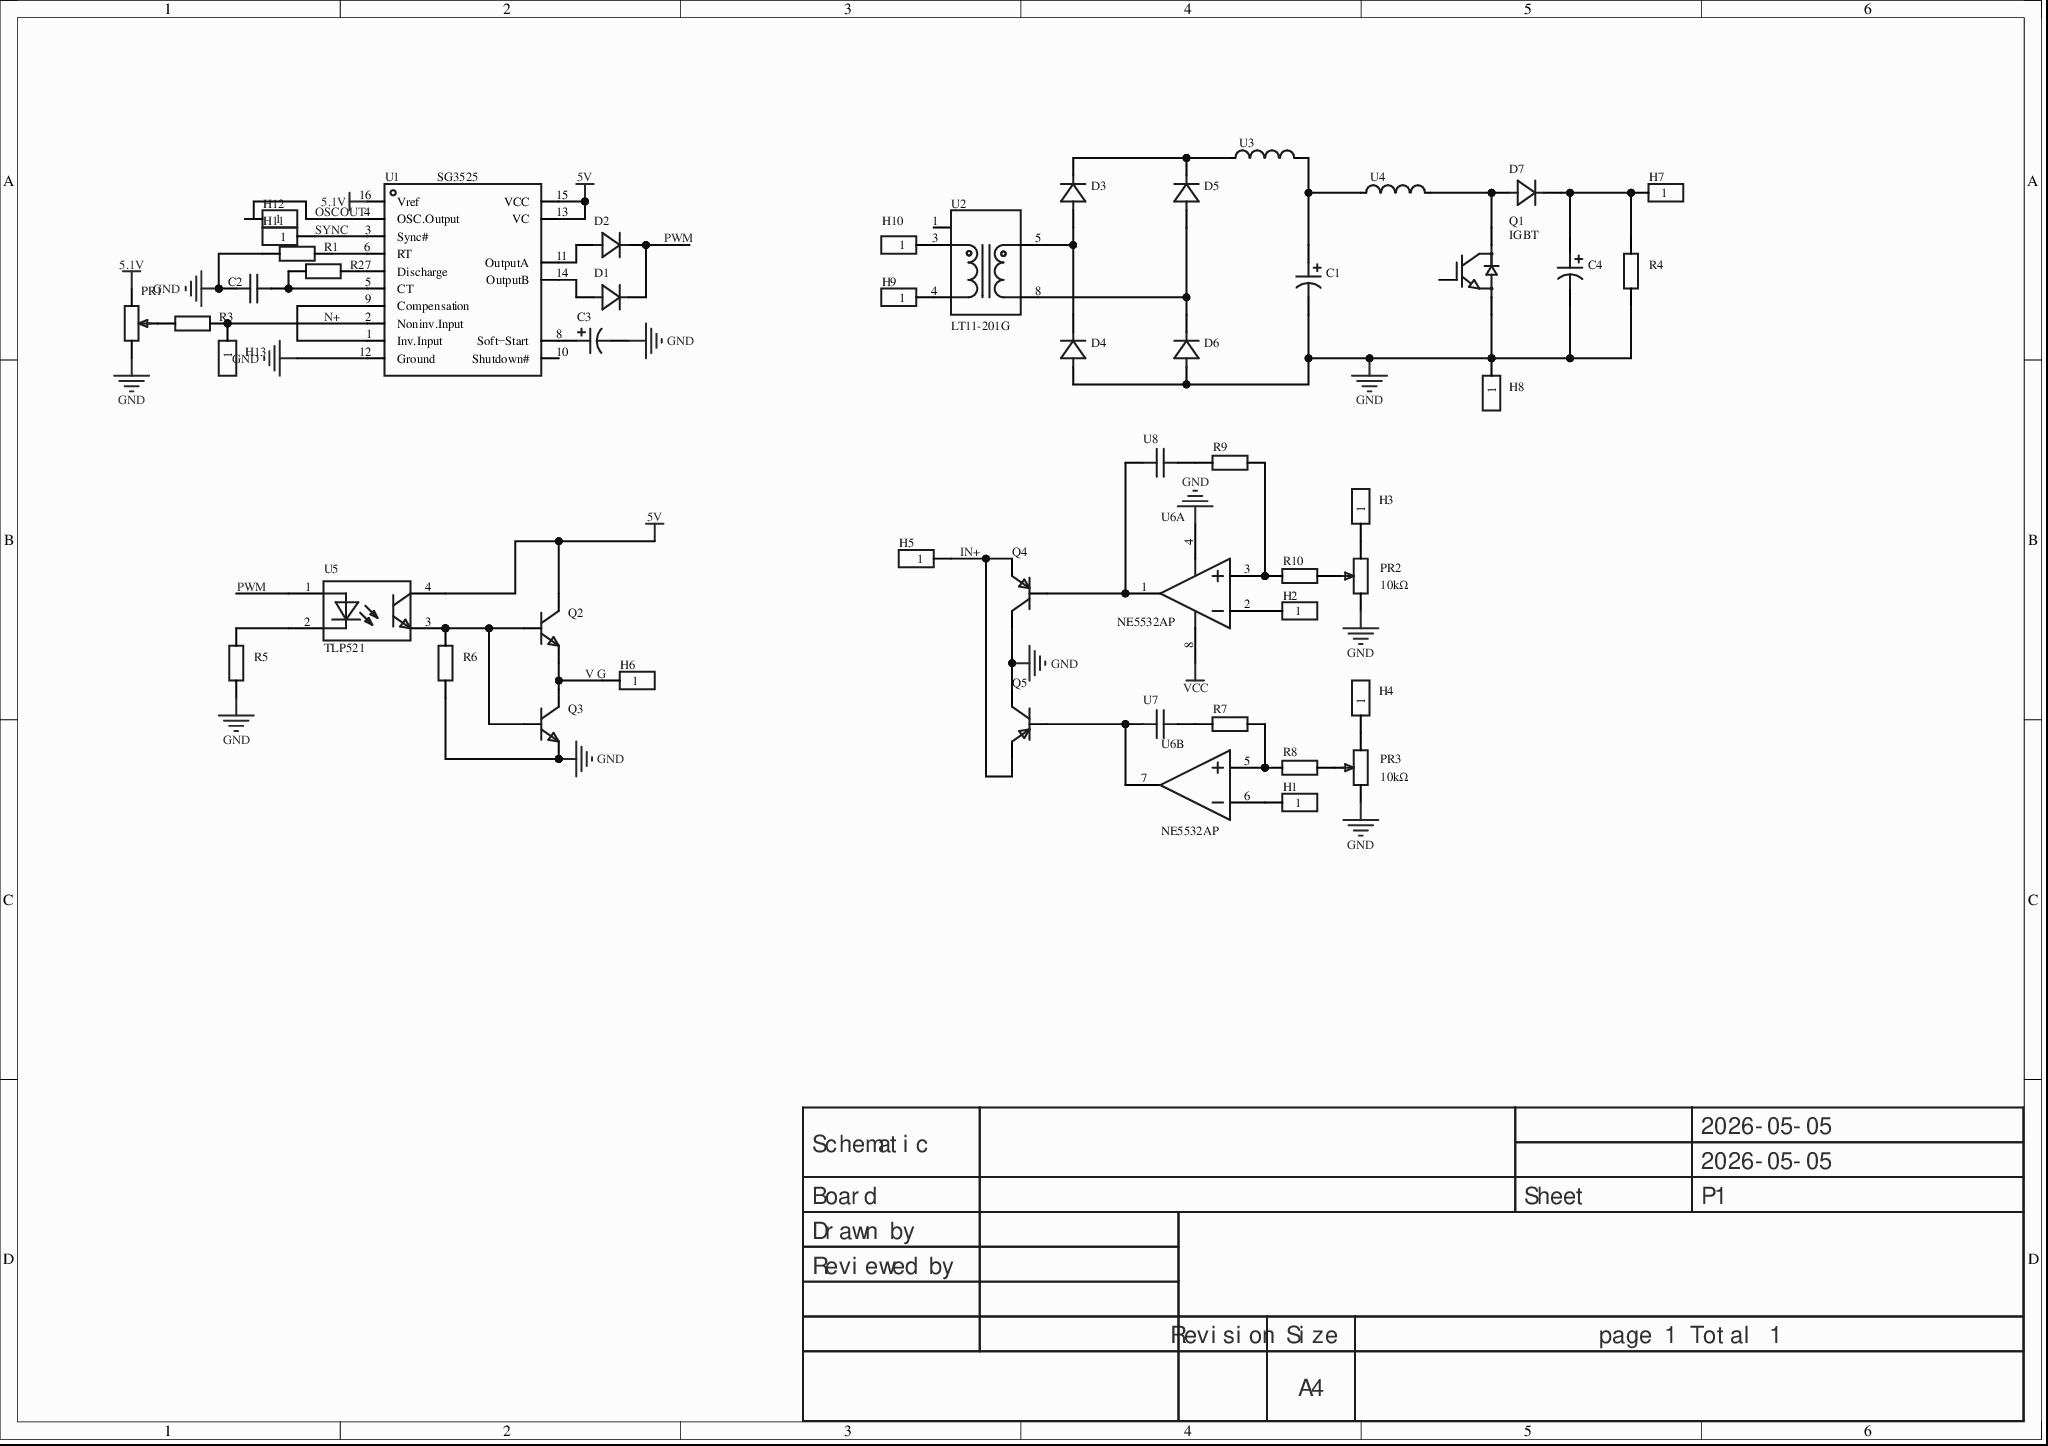
[diagram p0: MISC51628-3.schdoc]
# Altium project MISC51628-2.PrjPcb
1 sheet, 50 parts. Net scope: global (net labels, ports and power ports of the same name join across sheets).
Board file: MISC51628.pcbdoc

## Sheet MISC51628-3.schdoc
size 297 x 209 mm; Version: V1.0; @Project Name: MISC51628; @Update Date: 2026-05-05; @Create Date: 2026-05-05; @Board Name: MISC51628; @Create Time: 00:14:23; @Page Count: 1; @Page No: 1; @Schematic Name: MISC51628; @Update Time: 00:14:23; Size: A4

### Parts
C1  10uF  [CAP-TH_BD5.0-P2.00-D0.8-FD-10UF50VC110GL]  (value not drawn)
C2  100nF  [CAP-TH_L5.0-W2.5-P5.00-D1.0]  (value not drawn)
C3  10uF  [CAP-TH_BD5.0-P2.00-D0.8-FD-10UF50VC110GL]  (value not drawn)
C4  10uF  [CAP-TH_BD5.0-P2.00-D0.8-FD-10UF50VC110GL]  (value not drawn)
D1  (no value)  [DO_1N4007]
D2  (no value)  [DO_1N4007]
D3  (no value)  [DO_1N4007]
D4  (no value)  [DO_1N4007]
D5  (no value)  [DO_1N4007]
D6  (no value)  [DO_1N4007]
D7  (no value)  [DO_1N4007]
H1  (no value)  [HDR-TH_1P-V-M_XKB_X4611WV-01I-C28D40]
H2  (no value)  [HDR-TH_1P-V-M_XKB_X4611WV-01I-C28D40]
H3  (no value)  [HDR-TH_1P-V-M_XKB_X4611WV-01I-C28D40]
H4  (no value)  [HDR-TH_1P-V-M_XKB_X4611WV-01I-C28D40]
H5  (no value)  [HDR-TH_1P-V-M_XKB_X4611WV-01I-C28D40]
H6  (no value)  [HDR-TH_1P-V-M_XKB_X4611WV-01I-C28D40]
H7  (no value)  [HDR-TH_1P-V-M_XKB_X4611WV-01I-C28D40]
H8  (no value)  [HDR-TH_1P-V-M_XKB_X4611WV-01I-C28D40]
H9  (no value)  [HDR-TH_1P-V-M_XKB_X4611WV-01I-C28D40]
H10  (no value)  [HDR-TH_1P-V-M_XKB_X4611WV-01I-C28D40]
H11  (no value)  [HDR-TH_1P-V-M_XKB_X4611WV-01I-C28D40]
H12  (no value)  [HDR-TH_1P-V-M_XKB_X4611WV-01I-C28D40]
H13  (no value)  [HDR-TH_1P-V-M_XKB_X4611WV-01I-C28D40]
PR1  10kΩ  [R_3296]  (value not drawn)
PR2  10kΩ  [R_3296]
PR3  10kΩ  [R_3296]
Q1  IGBT  [TO-247-3_L15.9-W5.0-P5.44-L]
Q2  (no value)  [S8050_TO_92]
Q3  (no value)  [S8050_TO_92]
Q4  (no value)  [S8550P_SOT]
Q5  (no value)  [S8550P_SOT]
R1  10kΩ  [Res_1/8W]  (value not drawn)
R2  10kΩ  [Res_1/8W]  (value not drawn)
R3  10kΩ  [Res_1/8W]  (value not drawn)
R4  10kΩ  [Res_1/8W]  (value not drawn)
R5  10kΩ  [Res_1/8W]  (value not drawn)
R6  10kΩ  [Res_1/8W]  (value not drawn)
R7  10kΩ  [Res_1/8W]  (value not drawn)
R8  10kΩ  [Res_1/8W]  (value not drawn)
R9  10kΩ  [Res_1/8W]  (value not drawn)
R10  10kΩ  [Res_1/8W]  (value not drawn)
U1  SG3525  [DIP-16_L19.2-W6.6-P2.54-LS7.6-BL]
U2  LT11-201G  [XFMR-TH_LT13-201]
U3  Power inductor (SMD), CKST0502-10uH/M, 10uH, ±20%, 3A, package 5.7mm*5.1mm*2.0mm, Cenke, RoHS  [IND-SMD_L5.7-W5.1]  (value not drawn)
U4  Power inductor (SMD), CKST0502-10uH/M, 10uH, ±20%, 3A, package 5.7mm*5.1mm*2.0mm, Cenke, RoHS  [IND-SMD_L5.7-W5.1]  (value not drawn)
U5  TLP521  [SOP-4_L6.4-W4.6-P2.54-LS10.2-TL]
U6  NE5532AP  [PDIP-8_L9.6-W6.4-P2.54-LS7.6-BL]  (parts A,B of 2)
U7  100nF  [CAP-TH_L5.0-W2.5-P5.00-D1.0]  (value not drawn)
U8  100nF  [CAP-TH_L5.0-W2.5-P5.00-D1.0]  (value not drawn)

### Nets
5.1V: PR1.3 U1.16(Vref)
5V: Q2.3(C) U1.13(VC) U1.15(VCC) U5.4
GND: C1.2 C2.2 C3.2 C4.2 D4.2(A) D6.2(A) H8.1 PR1.1 PR2.3 PR3.3 Q1.3(E) Q3.1(E) Q4.3(C) Q5.3(C) R1.1 R4.1 R5.1 R6.1 U1.12(Ground) U6.4(V-)
VCC: U6.8(V+)
IN+: H5.1 Q4.2(E) Q5.2(E)
N+: H13.1 R3.2 U1.2(Noninv.Input)
OSCOUT: H12.1 U1.4(OSC.Output)
PWM: D1.1(K) D2.1(K) U5.1
SYNC: H11.1 U1.3(Sync#)
V G: H6.1 Q2.1(E) Q3.3(C)
NetC1_1: C1.1 U3.2 U4.1
NetC2_1: C2.1 R2.1 U1.5(CT)
NetC3_1: C3.1 U1.8(Soft−Start)
NetC4_1: C4.1 D7.1(K) H7.1 R4.2
NetD1_2: D1.2(A) U1.14(OutputB)
NetD2_2: D2.2(A) U1.11(OutputA)
NetD3_1: D3.1(K) D5.1(K) U3.1
NetD3_2: D3.2(A) D4.1(K) U2.5
NetD5_2: D5.2(A) D6.1(K) U2.8
NetD7_2: D7.2(A) Q1.2(C) U4.2
NetH1_1: H1.1 U6.6(IN_B-)
NetH2_1: H2.1 U6.2(IN_A-)
NetH3_1: H3.1 PR2.1
NetH4_1: H4.1 PR3.1
NetH9_1: H9.1 U2.4
NetH10_1: H10.1 U2.3
NetPR1_2: PR1.2 R3.1
NetPR2_2: PR2.2 R10.1
NetPR3_2: PR3.2 R8.1
NetQ2_2: Q2.2(B) Q3.2(B) R6.2 U5.3
NetQ4_1: Q4.1(B) U6.1(OUT_A) U8.2
NetQ5_1: Q5.1(B) U6.7(OUT_B) U7.2
NetR1_2: R1.2 U1.6(RT)
NetR2_2: R2.2 U1.7(Discharge)
NetR5_2: R5.2 U5.2
NetR7_1: R7.1 R8.2 U6.5(IN_B+)
NetR7_2: R7.2 U7.1
NetR9_1: R9.1 R10.2 U6.3(IN_A+)
NetR9_2: R9.2 U8.1
NetU1_1: U1.1(Inv.Input) U1.9(Compensation)

Not connected (* = marked no-connect by the designer): Q1 1(G); U1 10(Shutdown#); U2 1

### Notes on the sheet
- 2026-05-05
- Schematic
- Board
- Sheet
- P1
- Drawn by
- Reviewed by
- Revision
- Size
- A4
- page 1 Total 1

### Library data of the parts
C1 C4 = 10UF50VC110GL: Capacitance:10uF;Tolerance:±20%;Rated voltage:50V;Ripple current:120mA@100KHz;Equivalent series resistance(ESR):1.6Ω;; Manufacturer: Econd(米朗电子); Tolerance: ±20%; Voltage Rating: 50V; Equivalent Series Resistance(ESR): 1.6Ω; Pin Spacing: 2mm; Lifetime: 5000hrs@105℃; AddInBom: yes; Symbol: 10UF50VC110GL; Device: 10UF50VC110GL; LCSC Part Name: 10uF ±20% 50V; Supplier Part: C46867109; Manufacturer Part: 10UF50VC110GL; Supplier Footprint: 插件,D5xL11mm; JLCPCB Part Class: Extended Part; Datasheet: https://example.com/datasheet/10UF50VC110GL/49031974.html; Supplier: LCSC; Value: 10uF; Ripple Current: 120mA@100KHz; Diameter: 5mm; Height - Seated (Max): 11mm; Operating Temperature: -40℃~+105℃; ConvertToPcb: yes; FootprintName: CAP-TH_BD5.0-P2.00-D0.8-FD-10UF50VC110GL
C2 = 100nF: Symbol: 100NF_C9900015256; AddInBom: yes; ModelId: 08e3d7481fc7486bb1b263873f51e1e10819f05c4eef4c71ace90d822a990e87; ModelName: CAP-TH_BD5.0-W2.5-P5.08; ModelTransform: 224.652,98.425,0,0,0,0,-0.005,0,-137.795; Device: 100nF; LCSC Part Name: 100nF; SupplierPart: C9900015256; ManufacturerPart: 100nF; Supplier Footprint: CAP-TH_L5.0-W2.5-P5.00-D1.0; JLCPCB Part Class: Extended Part; Supplier: LCSC; ConvertToPcb: yes; FootprintName: CAP-TH_L5.0-W2.5-P5.00-D1.0
C3 = 10UF50VC110GL: Capacitance:10uF;Tolerance:±20%;Rated voltage:50V;Ripple current:120mA@100KHz;Equivalent series resistance(ESR):1.6Ω;; Manufacturer: Econd(米朗电子); AddInBom: yes; Tolerance: ±20%; Voltage Rating: 50V; Equivalent Series Resistance(ESR): 1.6Ω; Pin Spacing: 2mm; Lifetime: 5000hrs@105℃; Symbol: 10UF50VC110GL; Device: 10UF50VC110GL; LCSC Part Name: 10uF ±20% 50V; SupplierPart: C46867109; ManufacturerPart: 10UF50VC110GL; Supplier Footprint: 插件,D5xL11mm; JLCPCB Part Class: Extended Part; Datasheet: https://example.com/datasheet/10UF50VC110GL/49031974.html; Supplier: LCSC; ConvertToPcb: yes; FootprintName: CAP-TH_BD5.0-P2.00-D0.8-FD-10UF50VC110GL; Value: 10uF; Ripple Current: 120mA@100KHz; Diameter: 5mm; Height - Seated (Max): 11mm; Operating Temperature: -40℃~+105℃
D1-D3 = D_1N4007A: AddInBom: yes; ModelId: 6de1e9b71a0d4751b4e9df530304c1a30819f05c4eef4c71ace90d822a990e87; ModelName: DO-41_D2.4-L4.7-P8.70; ModelTransform: 373.9,94.4,232.29,0,0,0,0,0,-140; Symbol: D_1N4007; Device: D_1N4007A; Supplier Footprint: DO-41; ConvertToPcb: yes; FootprintName: DO_1N4007
D4-D7 = D_1N4007A: 3D Model: 6de1e9b71a0d4751b4e9df530304c1a30819f05c4eef4c71ace90d822a990e87; 3D Model Transform: 373.9,94.4,232.29,0,0,0,0,0,-140; AddInBom: yes; ModelName: DO-41_D2.4-L4.7-P8.70; Symbol: D_1N4007; Device: D_1N4007A; Supplier Footprint: DO-41; ConvertToPcb: yes; FootprintName: DO_1N4007
H1-H13 = HDR-M_2.54_1x1P: Symbol: HDR_1x1; ConvertToPcb: yes; ModelId: 95857080d3cc4057a19a22ccce05e1710819f05c4eef4c71ace90d822a990e87; ModelTransform: 78.74,79.1337,0,0,0,0,0,0,-110.236; Device: HDR-M_2.54_1x1P; AddInBom: yes; SupplierPart: C81276; Supplier Footprint: 插件; FootprintName: HDR-TH_1P-V-M_XKB_X4611WV-01I-C28D40; JLCPCB Part Class: Extended Part; ModelName: HDR-TH_1P-V-M_XKB_X4611WV-01I-C28D40
PR1 = R_3296: ConvertToPcb: yes; ModelId: b182808559bb43bda9e7de64b64134cb0819f05c4eef4c71ace90d822a990e87; ModelName: 3296W; ModelTransform: 373.98,188.96,590.49,180,0,0,0,0,-140; Symbol: R_3296; Device: R_3296; AddInBom: yes; Supplier Footprint: 直插; FootprintName: R_3296; Value: 10kΩ
PR2 PR3 = R_3296: 3D Model: b182808559bb43bda9e7de64b64134cb0819f05c4eef4c71ace90d822a990e87; 3D Model Transform: 373.98,188.96,590.49,180,0,0,0,0,-140; ConvertToPcb: yes; ModelName: 3296W; Symbol: R_3296; Device: R_3296; Supplier Footprint: 直插; Value: 10kΩ; AddInBom: yes; FootprintName: R_3296
Q1 = MLG40T65FDL-W: Uses advanced trench gate field-stop technology (Trench FS), collector-emitter breakdown voltage Vces=650V, collector current Ic=40A, with low conduction voltage drop and low turn-off loss, etc…; Manufacturer: minos(迈诺斯); AddInBom: yes; ModelId: 06d11a66e67643458860efec572770e60819f05c4eef4c71ace90d822a990e87; ModelTransform: 625.983,196.85,0,0,0,0,0,5.906,-196.85; Symbol: MLG40T65FDL-W; Device: MLG40T65FDL-W; Manufacturer Part: IGBT; LCSC Part Name: IGBT 650V 40A; SupplierPart: C54770473; Supplier Footprint: TO-3P; JLCPCB Part Class: Extended Part; Datasheet: https://example.com/datasheet/MLG40T65FDL-W/58189658.html; Supplier: LCSC; ConvertToPcb: yes; FootprintName: TO-247-3_L15.9-W5.0-P5.44-L; ModelName: TO-247-3_L15.9-W5.0-P5.44-L
Q2 Q3 = S8050_TO_NPN: ConvertToPcb: yes; ModelId: aafe8e06f2154e7c93506efd0d6632dd0819f05c4eef4c71ace90d822a990e87; ModelName: TO-92-3_L4.9-W3.7-P1.27-L; ModelTransform: 180.78,141.44,417.3,0,0,0,0,0,-200; Symbol: S8050_TO_NPN; Device: S8050_TO_NPN; AddInBom: yes; Supplier Footprint: TO-92; FootprintName: S8050_TO_92
Q4 Q5 = S8550_SOT_PNP: Symbol: PNP; ConvertToPcb: yes; ModelId: 9c0df02d6f3e44e889da37f3e5bf54960819f05c4eef4c71ace90d822a990e87; ModelName: SOT-23-3_L2.9-W1.4-P1.90-LS2.5-BR; ModelTransform: 98.43,114.17,37.91,0,0,0,0,0,0; Device: S8550_SOT_PNP; AddInBom: yes; Supplier Footprint: SOT-23; FootprintName: S8550P_SOT
R1-R3 = Res_AXIAL-1/8W: Symbol: Resistor; ConvertToPcb: yes; ModelId: b2b5ae7ae4c642178fe0039925c86a3f0819f05c4eef4c71ace90d822a990e87; ModelName: RES-TH_BD1.8-L3.2-P7.20-D0.4; ModelTransform: 282.86,66.88,253.09,0,0,0,0,0,-191; Device: Res_AXIAL-1/8W; AddInBom: yes; Supplier Footprint: 轴向引线; Value: 10kΩ; FootprintName: Res_1/8W
R4-R10 = Res_AXIAL-1/8W: Symbol: Resistor; 3D Model: b2b5ae7ae4c642178fe0039925c86a3f0819f05c4eef4c71ace90d822a990e87; 3D Model Transform: 282.86,66.88,253.09,0,0,0,0,0,-191; ConvertToPcb: yes; ModelName: RES-TH_BD1.8-L3.2-P7.20-D0.4; Device: Res_AXIAL-1/8W; Supplier Footprint: 轴向引线; Value: 10kΩ; AddInBom: yes; FootprintName: Res_1/8W
U1 = SG3525: Operating voltage: 8V~35V; switching frequency: 100Hz~500kHz; output current: 400mA; transistor withstand voltage: -;; Manufacturer: Gcore(扬州国芯); Symbol: SG3525_1; AddInBom: yes; ModelId: 36ad9a7692634580875d8a15b0e444ee0819f05c4eef4c71ace90d822a990e87; ModelName: DIP-16_L19.2-W6.6-H3.3-LS7.62-P2.54; ModelTransform: 755.904,311.8104,0,0,0,0,0,0,-118.11; Pd - Power Dissipation: 1000mW; Duty Cycle(Max): 49%; Topology: Totem pole; Device: SG3525; LCSC Part Name: PWM控制器; SupplierPart: C5157689; ManufacturerPart: SG3525; Supplier Footprint: DIP-16; JLCPCB Part Class: Extended Part; Datasheet: https://example.com/datasheet/SG3525/5796617.html; Supplier: LCSC; ConvertToPcb: yes; FootprintName: DIP-16_L19.2-W6.6-P2.54-LS7.6-BL; Isolation: -; Voltage - Supply: 8V~35V; Frequency - Switching: 100Hz~500kHz; Output Current: 400mA; Voltage - Breakdown: -; Features: Undervoltage protection (UVP); soft start; Operating Temperature: 0℃~+70℃; Working Mode: -; Output Voltage: -; Feedback System: -
U2 = LT11-201G: Transformer  Through-hole broadband carrier coupling transformer, high withstand voltage; Manufacturer: Linekey(立凯电控); AddInBom: yes; ModelId: 978c4cfc96044b13b294b69b1fbf46df0819f05c4eef4c71ace90d822a990e87; ModelTransform: 399.6055,451.1802,0,0,0,0,-0.002,0,-137.795; Symbol: LT11-201G; Device: LT11-201G; LCSC Part Name: 变压器; SupplierPart: C19274033; ManufacturerPart: LT11-201G; Supplier Footprint: 插件,11.4x10.1mm; JLCPCB Part Class: Extended Part; Datasheet: https://example.com/upload/public/pdf/source/20231201/8CB723A30866AEEAB4FA21B3FDB2AC71.pdf; Supplier: LCSC; ConvertToPcb: yes; FootprintName: XFMR-TH_LT13-201; ModelName: XFMR-TH_LT13-201
U3 U4 = 功率电感(贴片),CKST0502-10uH/M,10uH,±20%,3A,封装5.7mm*5.1mm*2.0mm,岑科,RoHS: AddInBom: yes; ModelId: ffd856615f974dd9b1ff3f65e3b3100d0819f05c4eef4c71ace90d822a990e87; ModelTransform: 224.409,200.787,0,0,0,0,0,-0.591,0; Symbol: Power inductor (SMD), CKST0502-10UH/M, 10UH, ±20%, 3A, package 5.7MM*5.1MM*2.0MM, Cenke, ROHS; Device: Power inductor (SMD), CKST0502-10uH/M, 10uH, ±20%, 3A, package 5.7mm*5.1mm*2.0mm, Cenke, RoHS; LCSC Part Name: 功率电感(贴片),CKST0502-10uH/M,10uH,±20%,3A,封装5.7mm*5.1mm*2.0mm,岑科,RoHS; SupplierPart: C9900015114; ManufacturerPart: 功率电感(贴片),CKST0502-10uH/M,10uH,±20%,3A,封装5.7mm*5.1mm*2.0mm,岑科,RoHS; Supplier Footprint: 功率电感(贴片),CKST0502-10uH/M,10uH,±20%,3A,封装5.7mm*5.1mm*2.0mm,岑科,RoHS; JLCPCB Part Class: Extended Part; Supplier: LCSC; ConvertToPcb: yes; FootprintName: IND-SMD_L5.7-W5.1; ModelName: IND-SMD_L5.7-W5.1
U5 = TLP521: AddInBom: yes; ModelId: 96de0c972fa141a0bf05d1bdcf0ddf4e0819f05c4eef4c71ace90d822a990e87; ModelName: SOP-4_L4.6-W6.5-H3.5-LS10.2_P2.54; ModelTransform: 181.102,401.574,0,270,0,0,0,0,0; Symbol: TLP521; Device: TLP521; LCSC Part Name: TLP521; SupplierPart: C9900005355; ManufacturerPart: TLP521; Supplier Footprint: SOP-4-2.54mm; JLCPCB Part Class: Extended Part; Supplier: LCSC; ConvertToPcb: yes; FootprintName: SOP-4_L6.4-W4.6-P2.54-LS10.2-TL
U6 = NE5532AP: Dual-channel, 30V, 10MHz, low-noise (6nV/√Hz) operational amplifier for audio applications; Manufacturer: TI(德州仪器); Relevance: []; AddInBom: yes; ModelId: 5dc2af053da0476fab11ee64b9a10a940819f05c4eef4c71ace90d822a990e87; ModelName: PDIP-8_L9.6-W6.4-P2.54-LS7.62-BL; ModelTransform: 377.952,309.842,0,0,0,0,0,0,-137.795; Symbol: NE5532AP; Device: NE5532AP; LCSC Part Name: NE5532AP; SupplierPart: C353150; ManufacturerPart: NE5532AP; Supplier Footprint: PDIP-8; JLCPCB Part Class: Extended Part; Supplier: LCSC; ConvertToPcb: yes; FootprintName: PDIP-8_L9.6-W6.4-P2.54-LS7.6-BL
U7 U8 = 100nF: Symbol: 100NF_C9900015256; 3D Model: 08e3d7481fc7486bb1b263873f51e1e10819f05c4eef4c71ace90d822a990e87; 3D Model Transform: 224.652,98.425,0,0,0,0,-0.005,0,-137.795; AddInBom: yes; ModelName: CAP-TH_BD5.0-W2.5-P5.08; Device: 100nF; LCSC Part Name: 100nF; Supplier Part: C9900015256; Manufacturer Part: 100nF; Supplier Footprint: CAP-TH_L5.0-W2.5-P5.00-D1.0; JLCPCB Part Class: Extended Part; Supplier: LCSC; ConvertToPcb: yes; FootprintName: CAP-TH_L5.0-W2.5-P5.00-D1.0